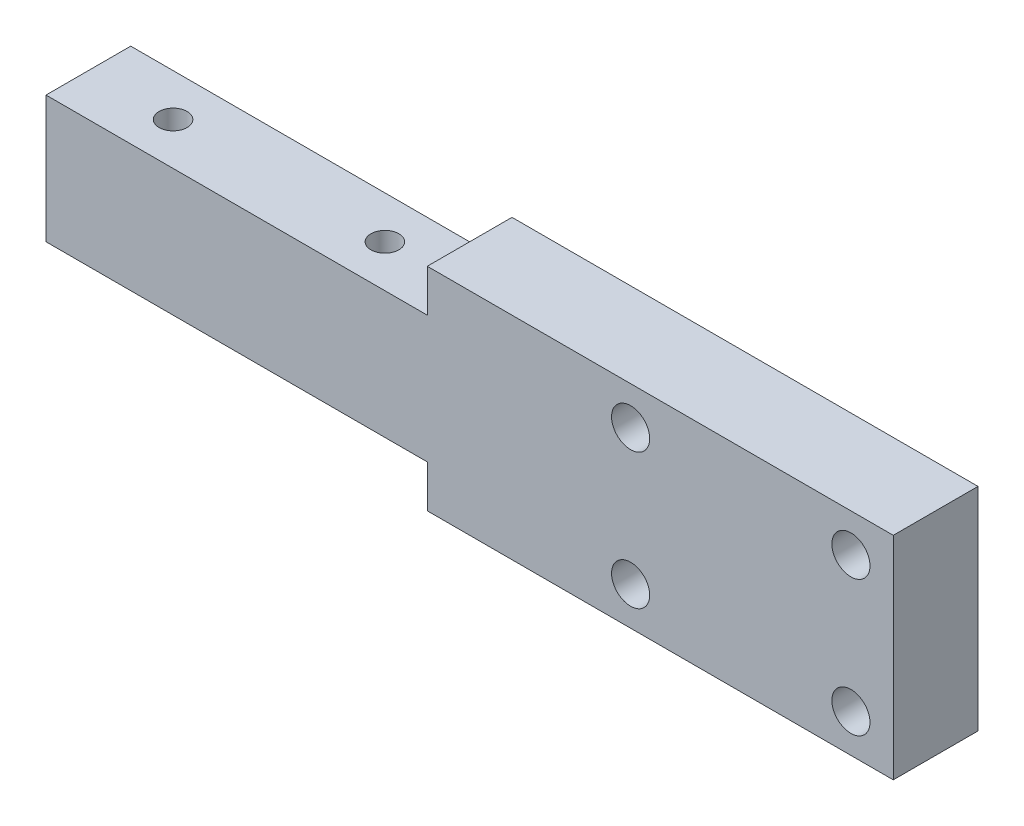
from build123d import *

# Parameters (mm, degrees)
SKETCH1_W                                        = 100
SKETCH1_H                                        = 25
BOSS_EXTRUDE1_DEPTH                              = 10
CUT_EXTRUDE1_DEPTH                               = 53.5
CUT_EXTRUDE1_DEPTH_BACK                          = 53.5
SKETCH2_W                                        = 45
SKETCH2_H                                        = 5
HOLE_FOR_SOCKET_HEAD_CAP_SCREW_TYPE1_D           = 4.5
HOLE_FOR_SOCKET_HEAD_CAP_SCREW_TYPE1_CBORE_D     = 8
HOLE_FOR_SOCKET_HEAD_CAP_SCREW_TYPE1_CBORE_DEPTH = 4.6
M4_TAPPED_HOLE1_D                                = 3.3


with BuildPart() as part:
    # Sketch1 → Boss-Extrude1 (new body)
    with BuildSketch(Plane.XY):
        Rectangle(SKETCH1_W, SKETCH1_H)
    extrude(amount=BOSS_EXTRUDE1_DEPTH)

    # Sketch2 → Cut-Extrude1 (cut, two sides: drawn at the far end of the back side and taken through both)
    with BuildSketch(Plane(origin=(0, 0, 0), x_dir=(-1, 0, 0), z_dir=(0, 0, -1)).offset(-CUT_EXTRUDE1_DEPTH_BACK)):
        with Locations((27.5, 10)):
            Rectangle(SKETCH2_W, SKETCH2_H)
        with Locations((27.5, -10)):
            Rectangle(SKETCH2_W, SKETCH2_H)
    extrude(amount=CUT_EXTRUDE1_DEPTH + CUT_EXTRUDE1_DEPTH_BACK, mode=Mode.SUBTRACT)

    # Hole for socket head cap screw, type1 (through all)
    with Locations(Plane(origin=(0, 0, 0), x_dir=(-1, 0, 0), z_dir=(0, 0, -1))):
        with Locations((-19, -8), (-19, 8), (-45, 8), (-45, -8)):
            CounterBoreHole(HOLE_FOR_SOCKET_HEAD_CAP_SCREW_TYPE1_D / 2, HOLE_FOR_SOCKET_HEAD_CAP_SCREW_TYPE1_CBORE_D / 2, HOLE_FOR_SOCKET_HEAD_CAP_SCREW_TYPE1_CBORE_DEPTH)

    # M4 Tapped Hole1 (through all)
    with Locations(Plane(origin=(0, 7.5, 0), x_dir=(1, 0, 0), z_dir=(0, 1, 0))):
        with Locations((-15, -5), (-40, -5)):
            Hole(M4_TAPPED_HOLE1_D / 2)


solid = part.part
